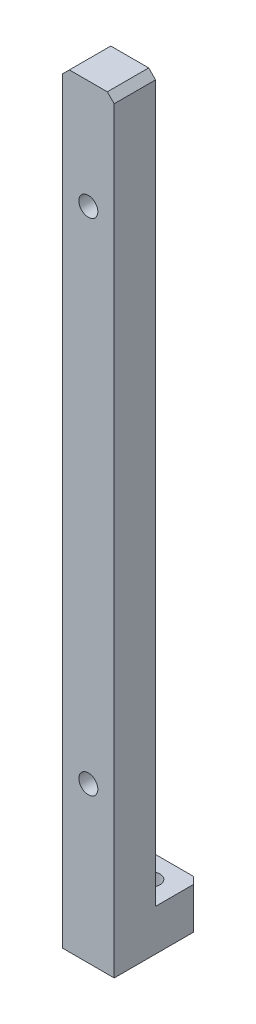
from build123d import *

# Parameters (mm, degrees)
BOSS_EXTRUDE1_DEPTH                                  = 15
CBORE_FOR_M5_HEXAGON_SOCKET_HEAD_CAP_SCR_D           = 5.5
CBORE_FOR_M5_HEXAGON_SOCKET_HEAD_CAP_SCR_CBORE_D     = 10
CBORE_FOR_M5_HEXAGON_SOCKET_HEAD_CAP_SCR_CBORE_DEPTH = 5.7
M5_CLEARANCE_HOLE1_D                                 = 5.5
CHAMFER1_SIZE                                        = 2


with BuildPart() as part:
    # Sketch1 → Boss-Extrude1 (new body)
    with BuildSketch(Plane(origin=(0, 0, 0), x_dir=(0, 0, -1), z_dir=(1, 0, 0))):
        Polygon((0, 0), (25, 0), (25, 12), (12, 12), (12, 221.5), (0, 221.5), align=None)
    extrude(amount=BOSS_EXTRUDE1_DEPTH)

    # CBORE for M5 Hexagon socket head cap screws1 (through all)
    with Locations(Plane(origin=(0, 0, -12), x_dir=(-1, 0, 0), z_dir=(0, 0, -1))):
        with Locations((-7.5, 45), (-7.5, 190)):
            CounterBoreHole(CBORE_FOR_M5_HEXAGON_SOCKET_HEAD_CAP_SCR_D / 2, CBORE_FOR_M5_HEXAGON_SOCKET_HEAD_CAP_SCR_CBORE_D / 2, CBORE_FOR_M5_HEXAGON_SOCKET_HEAD_CAP_SCR_CBORE_DEPTH)

    # M5 Clearance Hole1 (through all)
    with Locations(Plane(origin=(0, 0, 0), x_dir=(-1, 0, 0), z_dir=(0, -1, 0))):
        with Locations((-7.5, 18)):
            Hole(M5_CLEARANCE_HOLE1_D / 2)

    # Chamfer1
    chamfer1_edges = [part.edges().sort_by_distance(p)[0] for p in [
        (15, 6, -25),
        (15, 221.5, -6),
        (0, 221.5, -6),
        (0, 6, -25),
    ]]
    chamfer(chamfer1_edges, length=CHAMFER1_SIZE)


solid = part.part
